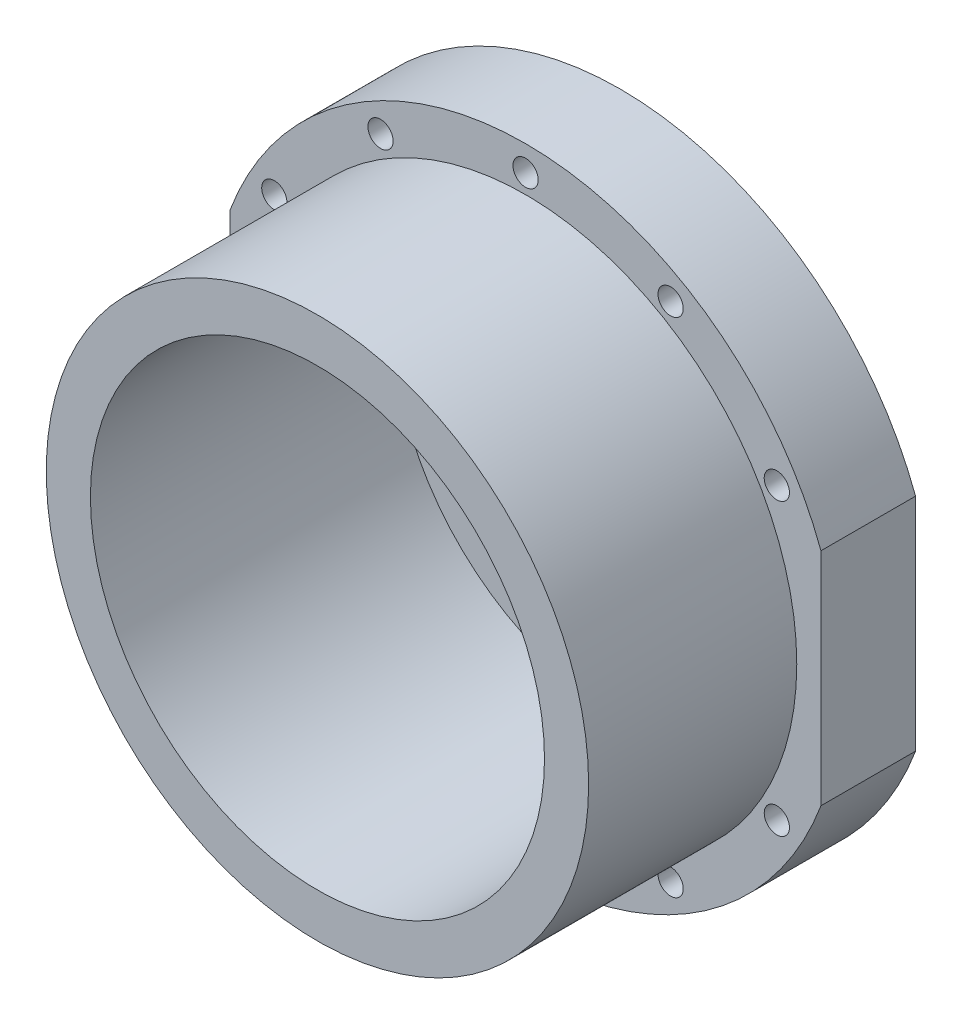
from build123d import *

# Parameters (mm, degrees)
SKETCH1_R           = 50
SKETCH1_R_2         = 36
BOSS_EXTRUDE1_DEPTH = 15
CUT_EXTRUDE1_START  = -48
CUT_EXTRUDE1_DEPTH  = 48
SKETCH4_R           = 40
SKETCH4_R_2         = 30
BOSS_EXTRUDE2_DEPTH = 5
SKETCH5_R           = 43
SKETCH5_R_2         = 36
BOSS_EXTRUDE3_DEPTH = 33
SKETCH6_R           = 2
CUT_EXTRUDE2_DEPTH  = 30


with BuildPart() as part:
    # Sketch1 → Boss-Extrude1 (new body)
    with BuildSketch(Plane.XY):
        Circle(SKETCH1_R)
        Circle(SKETCH1_R_2, mode=Mode.SUBTRACT)
    extrude(amount=BOSS_EXTRUDE1_DEPTH)

    # Sketch2 → Cut-Extrude1 (cut)
    with BuildSketch(Plane.XY.offset(15).offset(CUT_EXTRUDE1_START)):
        with BuildLine():
            Line((-46.835, 17.506649451), (-46.835, -17.506649451))
            ThreePointArc((-46.835, -17.506649451), (-50, 0), (-46.835, 17.506649451))
        make_face()
        with BuildLine():
            Line((46.835, 17.506649451), (46.835, -17.506649451))
            ThreePointArc((46.835, -17.506649451), (50, 0), (46.835, 17.506649451))
        make_face()
    extrude(amount=CUT_EXTRUDE1_DEPTH, mode=Mode.SUBTRACT)

    # Sketch4 → Boss-Extrude2 (add)
    with BuildSketch(Plane(origin=(0, 0, 0), x_dir=(-1, 0, 0), z_dir=(0, 0, -1))):
        with Locations(Location((0, 0, 0), (0, 0, 180))):
            Circle(SKETCH4_R)
        Circle(SKETCH4_R_2, mode=Mode.SUBTRACT)
    extrude(amount=BOSS_EXTRUDE2_DEPTH)

    # Sketch5 → Boss-Extrude3 (add)
    with BuildSketch(Plane.XY.offset(15)):
        Circle(SKETCH5_R)
        Circle(SKETCH5_R_2, mode=Mode.SUBTRACT)
    extrude(amount=BOSS_EXTRUDE3_DEPTH)

    # Sketch6 → Cut-Extrude2 (cut)
    with BuildSketch(Plane.XY.offset(15)):
        with Locations((0, 46)):
            Circle(SKETCH6_R)
        with Locations((39.837168574, -23)):
            Circle(SKETCH6_R)
        with Locations((23, 39.837168574)):
            Circle(SKETCH6_R)
        with Locations((39.837168574, 23)):
            Circle(SKETCH6_R)
        with Locations((-23, 39.837168574)):
            Circle(SKETCH6_R)
        with Locations((-39.837168574, 23)):
            Circle(SKETCH6_R)
        with Locations((23, -39.837168574)):
            Circle(SKETCH6_R)
        with Locations((0, -46)):
            Circle(SKETCH6_R)
        with Locations((-23, -39.837168574)):
            Circle(SKETCH6_R)
        with Locations((-39.837168574, -23)):
            Circle(SKETCH6_R)
    extrude(amount=-CUT_EXTRUDE2_DEPTH, mode=Mode.SUBTRACT)


solid = part.part
